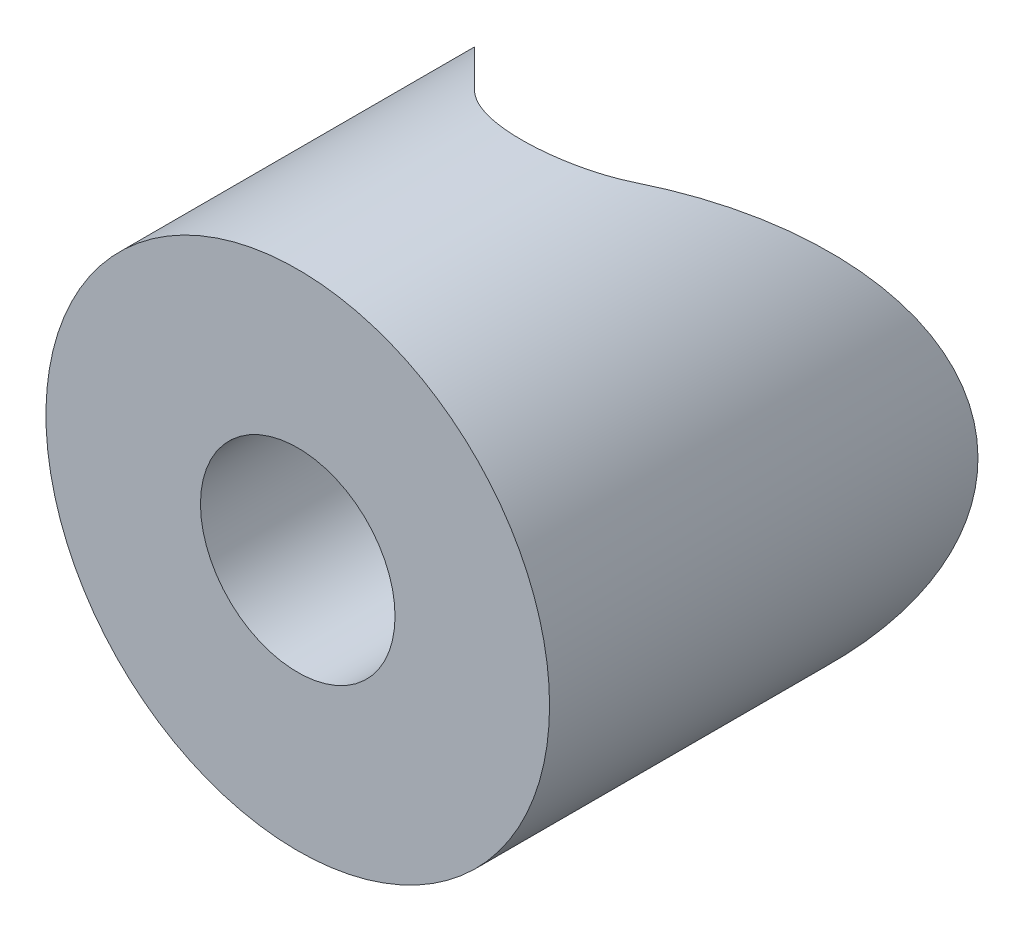
SolidWorks part; units mm, degrees
material "1023 碳钢板 (SS)"
ref_plane "Front Plane" through (0, 0, 0) normal (0, 0, 1) x (1, 0, 0)
ref_plane "Top Plane" through (0, 0, 0) normal (0, 1, 0) x (1, 0, 0)
ref_plane "Right Plane" through (0, 0, 0) normal (1, 0, 0) x (0, 0, -1)
sketch "Sketch1" plane through (0, 0, 0) normal (0, 0, 1) x (1, 0, 0)
  circle A0 centre (0, 0) radius 11
  dimension "D1" = 22
extrude "Boss-Extrude1" add sketch "Sketch1" along normal blind 19
hole_wizard "M10 Tapped Hole1" positions "Sketch2" profile "Sketch3" tap size "M10" standard "GB"
sketch "Sketch2" plane through (0, 0, 19) normal (0, 0, 1) x (1, 0, 0)
  point P0 (0, 0)
sketch "Sketch3" plane through (0, 0, 19) normal (1, 0, 0) x (0, -1, 0)
  line L0 (0, 0) -> (0, 27.0537)
  line L1 (0, 27.0537) -> (4.25, 24.5)
  line L2 (4.25, 24.5) -> (4.25, 0)
  line L5 (4.25, 0) -> (0, 0)
  line L10 (0, 27.0537) -> (-4.25, 24.5) construction
  line L11 (0, -6.35) -> (0, 107.95) construction
  dimension "螺纹孔钻头直径" = 8.5
  dimension "螺纹孔钻头深度" = 24.5
  dimension "导头角度" = 118
cosmetic thread "CosmeticThread Hole thread1" parameters "D1"=20, "D2"=10
sketch "Sketch4" plane through (0, 0, 0) normal (0, 1, 0) x (1, 0, 0)
  line L0 (3.5355, -7.7487) -> (28.2843, 17)
  line L1 (-3.5355, -7.7487) -> (-28.2843, 17)
  line L2 (28.2843, 17) -> (0, 45.2843)
  line L3 (-28.2843, 17) -> (0, 45.2843)
  line L4 (-28.2843, 17) -> (28.2843, 17) construction
  line L5 (11, 0) -> (-11, 0) construction
  line L6 (-11, -19) -> (11, -19) construction
  arc A0 (-3.5355, -7.7487) -> (3.5355, -7.7487) centre (0, -4.2132) ccw
  point P11 (0, -11.2843)
  dimension "D4" = 5
  dimension "D1" = 40
  dimension "D2" = 40
  dimension "D3" = 36
extrude "Cut-Extrude1" cut sketch "Sketch4" against normal mid plane 25
